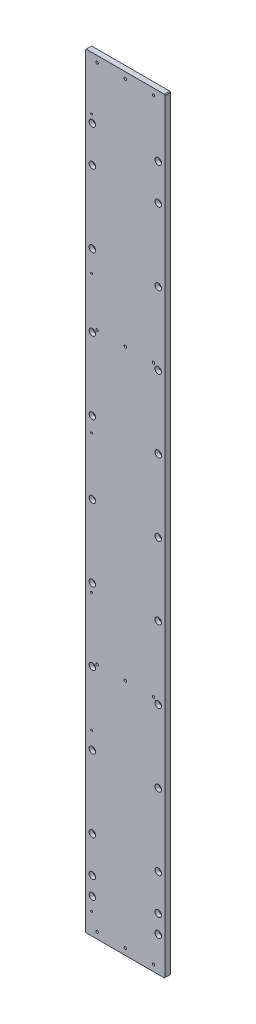
from build123d import *

# Parameters (mm, degrees)
SKETCH_1_W                    = 220
SKETCH_1_H                    = 2115
EXTRUDE_1_DEPTH               = 15
CHAMFER_1_SIZE                = 2
HOLE_WIZARD_M8_1_D            = 6.8
HOLE_WIZARD_M8_1_DEPTH        = 22.25
HOLE_WIZARD_M8_1_TIP          = 2.042926105
HOLE_WIZARD_M10_1_D           = 11
HOLE_WIZARD_M10_1_CBORE_D     = 18
HOLE_WIZARD_M10_1_CBORE_DEPTH = 10.6
HOLE_WIZARD_M6_2_D            = 5


with BuildPart() as part:
    # 草图1 → 凸台-拉伸1 (new body)
    with BuildSketch(Plane.XY):
        with Locations((110, 1057.5)):
            Rectangle(SKETCH_1_W, SKETCH_1_H)
    extrude(amount=EXTRUDE_1_DEPTH)

    # 倒角1
    chamfer_1_edges = [part.edges().sort_by_distance(p)[0] for p in [
        (220, 0, 7.5),
        (0, 0, 7.5),
        (0, 2115, 7.5),
        (220, 2115, 7.5),
    ]]
    chamfer(chamfer_1_edges, length=CHAMFER_1_SIZE)

    # M8 螺纹孔1
    with Locations(Plane.XY.offset(15)):
        with Locations((32, 2097.5), (32, 1457.5), (32, 657.5), (32, 17.5), (110, 2097.5), (110, 1457.5), (110, 657.5), (110, 17.5), (188, 2097.5), (188, 1457.5), (188, 657.5), (188, 17.5)):
            Hole(HOLE_WIZARD_M8_1_D / 2, depth=HOLE_WIZARD_M8_1_DEPTH)
            with Locations((0, 0, -(HOLE_WIZARD_M8_1_DEPTH + HOLE_WIZARD_M8_1_TIP / 2))):  # 118° drill point
                Cone(0, HOLE_WIZARD_M8_1_D / 2, HOLE_WIZARD_M8_1_TIP, mode=Mode.SUBTRACT)

    # M10 六角凹头螺钉的柱形沉头孔1 (through all)
    with Locations(Plane.XY.offset(15)):
        with Locations((19, 1946), (201, 1946), (19, 1846), (201, 1846), (19, 1646), (201, 1646), (19, 1446), (201, 1446), (19, 1246), (201, 1246), (19, 1046), (201, 1046), (19, 846), (201, 846), (19, 646), (201, 646), (19, 446), (201, 446), (19, 246), (201, 246), (19, 146), (201, 146), (19, 96), (201, 96)):
            CounterBoreHole(HOLE_WIZARD_M10_1_D / 2, HOLE_WIZARD_M10_1_CBORE_D / 2, HOLE_WIZARD_M10_1_CBORE_DEPTH)

    # M6 螺纹孔2 (through all)
    with Locations(Plane.XY.offset(15)):
        with Locations((16.75, 58.707106781), (16.75, 492.141421356), (16.75, 822.147106781), (16.75, 1203.867106781), (16.75, 1585.587106781), (16.75, 1967.307106781)):
            Hole(HOLE_WIZARD_M6_2_D / 2)


solid = part.part
